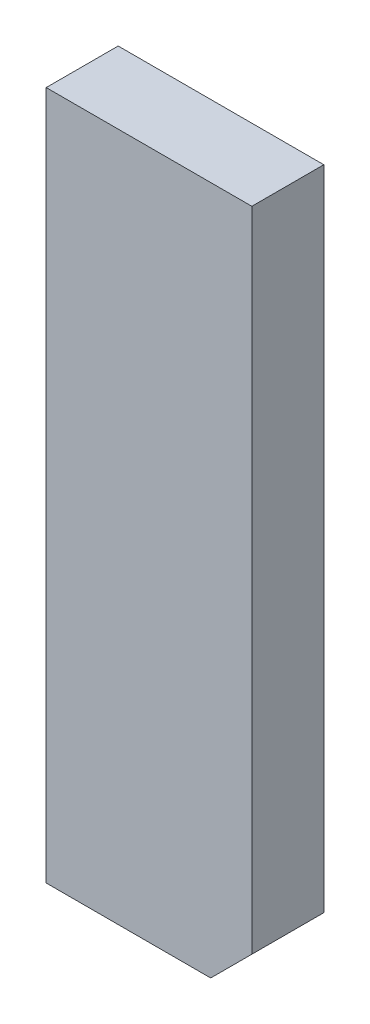
SolidWorks part; units mm, degrees
ref_plane "Front Plane" through (0, 0, 0) normal (0, 0, 1) x (1, 0, 0)
ref_plane "Top Plane" through (0, 0, 0) normal (0, 1, 0) x (1, 0, 0)
ref_plane "Right Plane" through (0, 0, 0) normal (1, 0, 0) x (0, 0, -1)
sketch "Sketch1" plane through (0, 0, 0) normal (0, 0, 1) x (1, 0, 0)
  line L1 (0, 0) -> (100, 0)
  line L2 (0, 0) -> (0, -335)
  line L3 (0, -335) -> (100, -335)
  line L4 (100, 0) -> (100, -335)
  dimension "D1" = 335
  dimension "D2" = 100
extrude "Boss-Extrude1" add sketch "Sketch1" along normal blind 35
chamfer "Chamfer1" distance 20 angle 45 1 edges at (100, -335, 17.5)
